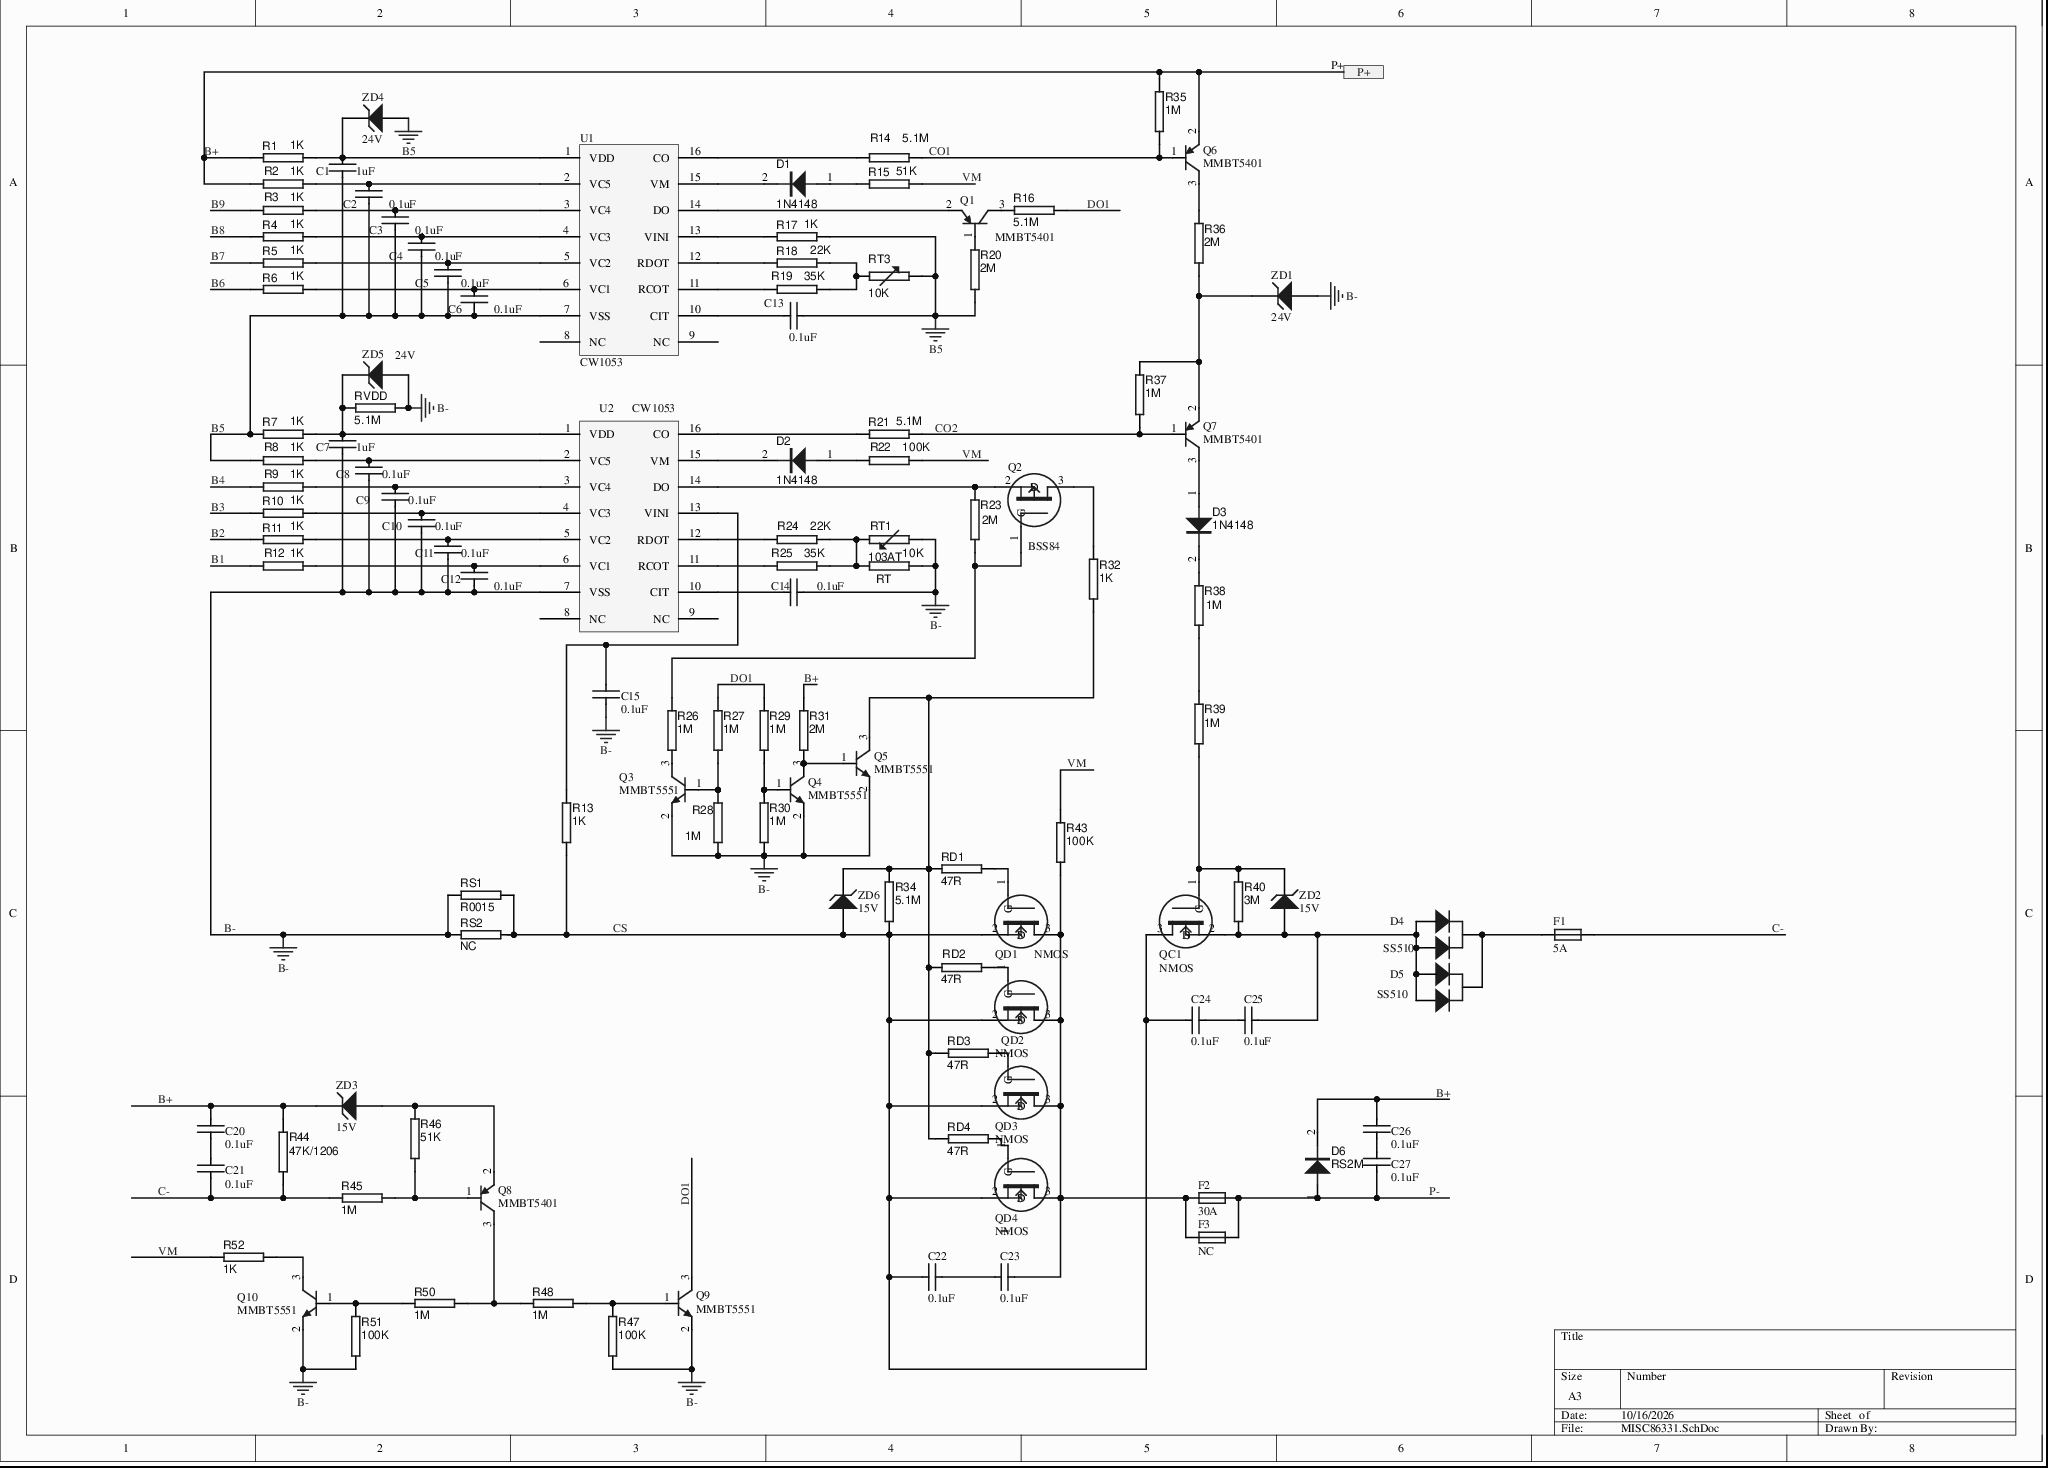
[diagram p0: MISC86331.SchDoc]
# Altium project MISC86331.PrjPcb
1 sheet, 113 parts. Net scope: flat (ports and power ports of the same name join across sheets).
Board file: MISC86331.PcbDoc

## Sheet MISC86331.SchDoc
size A3; SheetNumber: 1; SheetTotal: 1

### Parts
C1  1uF  [CAP0805]
C2  0.1uF  [C0603A]
C3  0.1uF  [C0603A]
C4  0.1uF  [C0603A]
C5  0.1uF  [C0603A]
C6  0.1uF  [C0603A]
C7  1uF  [CAP0805]
C8  0.1uF  [C0603A]
C9  0.1uF  [C0603A]
C10  0.1uF  [C0603A]
C11  0.1uF  [C0603A]
C12  0.1uF  [C0603A]
C13  0.1uF  [C0603A]
C14  0.1uF  [C0603A]
C15  0.1uF  [C0603A]
C20  0.1uF  [C0603A]
C21  0.1uF  [C0603A]
C22  0.1uF  [C0603A]
C23  0.1uF  [C0603A]
C24  0.1uF  [C0603A]
C25  0.1uF  [C0603A]
C26  0.1uF  [C0603A]
C27  0.1uF  [C0603A]
D1  1N4148  [SOD323]
D2  1N4148  [SOD323]
D3  1N4148  [SOD323]
D4  SS510  [TO-252-A]
D5  SS510  [TO-252-A]
D6  RS2M  [SMB-1]
F1  5A  [R1206]
F2  30A  [R1206]
F3  NC  [2410]
Q1  MMBT5401  [SOT-23-3]
Q2  BSS84  [SOT-23-3]
Q3  MMBT5551  [SOT-23-3]
Q4  MMBT5551  [SOT-23-3]
Q5  MMBT5551  [SOT-23-3]
Q6  MMBT5401  [SOT-23-3]
Q7  MMBT5401  [SOT-23-3]
Q8  MMBT5401  [SOT-23-3]
Q9  MMBT5551  [SOT-23-3]
Q10  MMBT5551  [SOT-23-3]
QC1  NMOS  [TO-252-A]
QD1  NMOS  [TO-252-A]
QD2  NMOS  [TO-252-A]
QD3  NMOS  [TO-252-A]
QD4  NMOS  [TO-252-A]
R1  1K  [RES0805]
R2  1K  [RES0603]
R3  1K  [RES0603]
R4  1K  [RES0603]
R5  1K  [RES0603]
R6  1K  [RES0603]
R7  1K  [RES0805]
R8  1K  [RES0603]
R9  1K  [RES0603]
R10  1K  [RES0603]
R11  1K  [RES0603]
R12  1K  [RES0603]
R13  1K  [R0603A]
R14  5.1M  [R0603A]
R15  51K  [R0603A]
R16  5.1M  [R0603A]
R17  1K  [R0603A]
R18  22K  [R0603A]
R19  35K  [R0603A]
R20  2M  [R0603A]
R21  5.1M  [R0603A]
R22  100K  [R0603A]
R23  2M  [R0603A]
R24  22K  [R0603A]
R25  35K  [R0603A]
R26  1M  [R0603A]
R27  1M  [R0603A]
R28  1M  [R0603A]
R29  1M  [R0603A]
R30  1M  [R0603A]
R31  2M  [R0603A]
R32  1K  [R0603A]
R34  5.1M  [R0603A]
R35  1M  [R0603A]
R36  2M  [R0603A]
R37  1M  [R0603A]
R38  1M  [R0603A]
R39  1M  [R0603A]
R40  3M  [R0603A]
R43  100K  [R0603A]
R44  47K/1206  [R1206]
R45  1M  [R0603A]
R46  51K  [R0603A]
R47  100K  [R0603A]
R48  1M  [R0603A]
R50  1M  [R0603A]
R51  100K  [R0603A]
R52  1K  [R0603A]
RD1  47R  [R0603A]
RD2  47R  [R0603A]
RD3  47R  [R0603A]
RD4  47R  [R0603A]
RS1  R0015  [2512]
RS2  NC  [2512]
RT  10K  [R0603A]
RT1  103AT  [WK]
RT3  10K  [R0603A]
RVDD  5.1M  [R0603A]
U1  CW1053  [SO-16]
U2  CW1053  [SO-16]
ZD1  24V  [SOD323]
ZD2  15V  [SOD323]
ZD3  15V  [SOD323]
ZD4  24V  [SOD323]
ZD5  24V  [SOD323]
ZD6  15V  [SOD323]

### Ports
P+

### Nets
B5: C1.2 C2.2 C3.2 C4.2 C5.2 C6.2 C13.2 R7.1 R8.1 R17.2 R20.1 RT3.2 U1.7(VSS) ZD4.1(A)
B-: C7.2 C8.2 C9.2 C10.2 C11.2 C12.2 C14.2 C15.1 Q3.2 Q4.2 Q5.2 Q9.2 Q10.2 R28.1 R30.1 R47.2 R51.2 RS1.1 RS2.1 RT.2 RT1.1 RVDD.1 U2.7(VSS) ZD1.1(A) ZD5.1(A)
B1: R12.1
B2: R11.2
B3: R10.1
B4: R9.1
B6: R6.1
B7: R5.1
B8: R4.1
B9: R3.1
B+: C20.1 C26.2 D6.2(K) Q6.2(E) R1.1 R2.1 R31.2 R35.2 R44.2 ZD3.2(K) ; port P+
C-: C21.2 F1.2 R44.1 R45.2
CO1: Q6.1(B) R14.2 R35.1
CO2: Q7.1(B) R21.2 R37.1
CS: C22.2 C24.2 QC1.3(D) QD1.2(S) QD2.2(S) QD3.2(S) QD4.2(S) R13.2 R34.1 RS1.2 RS2.2 ZD6.1(A)
DO1: Q9.3(C) R16.1 R27.2 R29.1
P-: C27.1 D6.1(A) F2.2 F3.2
VM: R15.2 R22.2 R43.2 R52.1
NetC1_1: C1.1 R1.2 U1.1(VDD) ZD4.2(K)
NetC2_1: C2.1 R2.2 U1.2(VC5)
NetC3_1: C3.1 R3.2 U1.3(VC4)
NetC4_1: C4.1 R4.2 U1.4(VC3)
NetC5_1: C5.1 R5.2 U1.5(VC2)
NetC6_1: C6.1 R6.2 U1.6(VC1)
NetC7_1: C7.1 R7.2 RVDD.2 U2.1(VDD) ZD5.2(K)
NetC8_1: C8.1 R8.2 U2.2(VC5)
NetC9_1: C9.1 R9.2 U2.3(VC4)
NetC10_1: C10.1 R10.2 U2.4(VC3)
NetC11_1: C11.1 R11.1 U2.5(VC2)
NetC12_1: C12.1 R12.2 U2.6(VC1)
NetC13_1: C13.1 U1.10(CIT)
NetC14_1: C14.1 U2.10(CIT)
NetC15_2: C15.2 R13.1 U2.13(VINI)
NetC20_2: C20.2 C21.1
NetC22_1: C22.1 C23.2
NetC23_1: C23.1 F2.1 F3.1 QD1.3(D) QD2.3(D) QD3.3(D) QD4.3(D) R43.1
NetC24_1: C24.1 C25.2
NetC25_1: C25.1 D4.1(A) D4.2(A) D5.1(A) D5.2(A) QC1.2(S) R40.1 ZD2.1(A)
NetC26_1: C26.1 C27.2
NetD1_1: D1.1(A) R15.1
NetD1_2: D1.2(K) U1.15(VM)
NetD2_1: D2.1(A) R22.1
NetD2_2: D2.2(K) U2.15(VM)
NetD3_1: D3.1(A) Q7.3(C)
NetD3_2: D3.2(K) R38.1
NetD4_3: D4.3(K) D5.3(K) F1.1
NetQ1_1: Q1.1(B) R20.2
NetQ1_2: Q1.2(E) U1.14(DO)
NetQ1_3: Q1.3(C) R16.2
NetQ2_1: Q2.1(G) R23.2 R26.1
NetQ2_2: Q2.2(S) R23.1 U2.14(DO)
NetQ2_3: Q2.3(D) R32.2
NetQ3_1: Q3.1(B) R27.1 R28.2
NetQ3_3: Q3.3(C) R26.2
NetQ4_1: Q4.1(B) R29.2 R30.2
NetQ4_3: Q4.3(C) Q5.1(B) R31.1
NetQ5_3: Q5.3(C) R32.1 R34.2 RD1.2 RD2.2 RD3.2 RD4.2 ZD6.2(K)
NetQ6_3: Q6.3(C) R36.1
NetQ7_2: Q7.2(E) R36.2 R37.2 ZD1.2(K)
NetQ8_1: Q8.1(B) R45.1 R46.2
NetQ8_2: Q8.2(E) R46.1 ZD3.1(A)
NetQ8_3: Q8.3(C) R48.2 R50.1
NetQ9_1: Q9.1(B) R47.1 R48.1
NetQ10_1: Q10.1(B) R50.2 R51.1
NetQ10_3: Q10.3(C) R52.2
NetQC1_1: QC1.1(G) R39.1 R40.2 ZD2.2(K)
NetQD1_1: QD1.1(G) RD1.1
NetQD2_1: QD2.1(G) RD2.1
NetQD3_1: QD3.1(G) RD3.1
NetQD4_1: QD4.1(G) RD4.1
NetR14_1: R14.1 U1.16(CO)
NetR17_1: R17.1 U1.13(VINI)
NetR18_1: R18.1 U1.12(RDOT)
NetR18_2: R18.2 R19.2 RT3.1
NetR19_1: R19.1 U1.11(RCOT)
NetR21_1: R21.1 U2.16(CO)
NetR24_1: R24.1 U2.12(RDOT)
NetR24_2: R24.2 R25.2 RT.1 RT1.2
NetR25_1: R25.1 U2.11(RCOT)
NetR38_2: R38.2 R39.2

Not connected (* = marked no-connect by the designer): U1 8(NC) 9(NC); U2 8(NC) 9(NC)

### Notes on the sheet
- P+

### Library data of the parts
C1-C15 C20-C27 = CAP
D1-D3 D6 = DIODE
D4 D5 = MBR10100DCT: SMD dual common-cathode diode
F1-F3 = FUSE
Q1 Q6-Q8 = PNP: PNP Bipolar Transistor; Published: 8-Jun-2000; LatestRevisionDate: 29-May-2009; LatestRevisionNote: IPC-7351 Footprint Added.; PackageVersion: Aug-1999; PackageReference: SOT-23B; PackageDescription: 3-Pin SOT-23 Package 0.95 mm Pitch, 2.4 mm Lead Span; Publisher: Altium Limited
Q2 = PMOS
Q3-Q5 Q9 Q10 = NPN: NPN Bipolar Transistor; Published: 8-Jun-2000; LatestRevisionDate: 17-Jul-2002; LatestRevisionNote: Re-released for DXP Platform.; PackageReference: TO-226-AA; PackageDescription: TO, Flat Index; 3 In-Line, Axial Leads; Body Dia. 4.8mm; Leads 0.55 x 0.51 mm (max); Code_JEDEC: TO-226-AA; Publisher: Altium Limited
R1-R32 R34-R40 R43-R48 R50-R52 RD1-RD4 RS1 RS2 RT RVDD = RES1: RES
RT1 RT3 = RES2: RES
ZD1-ZD6 = D Zener: Zener Diode; Published: 8-Jun-2000; LatestRevisionDate: 17-Jul-2002; LatestRevisionNote: Re-released for DXP Platform.; PackageReference: DIODE-0.7; PackageDescription: Diode, Thru-Hole; 2 Leads; 0.7 in Pin Spacing; Publisher: Altium Limited